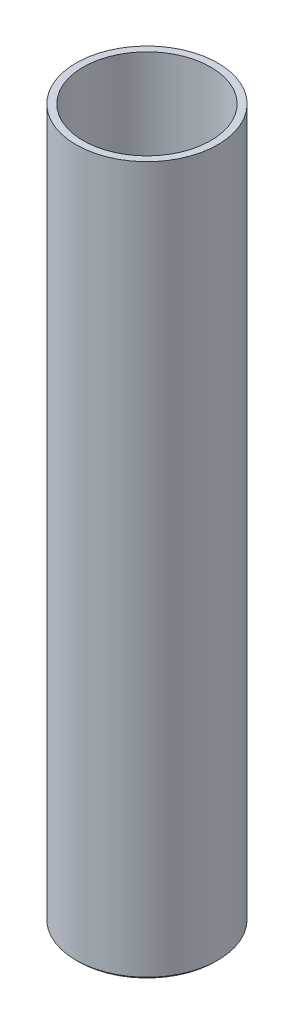
from build123d import *

# Parameters (mm, degrees)
SKETCH1_R           = 15
BOSS_EXTRUDE1_DEPTH = 150
SKETCH3_W           = 13.5
SKETCH3_H           = 147.5
SKETCH3_H_2         = 0.5
CHAMFER1_SIZE       = 0.5


with BuildPart() as part:
    # Sketch1 → Boss-Extrude1 (new body)
    with BuildSketch(Plane(origin=(0, 0, 0), x_dir=(1, 0, 0), z_dir=(0, 1, 0))):
        with Locations(Location((0, 0, 0), (0, 0, 270))):
            Circle(SKETCH1_R)
    extrude(amount=BOSS_EXTRUDE1_DEPTH)

    # Sketch3 → Cut-Revolve1 (revolve, cut)
    with BuildSketch(Plane.XY, mode=Mode.PRIVATE) as cut_revolve1_sk:
        with Locations((6.75, 76.25)):
            Rectangle(SKETCH3_W, SKETCH3_H)
        with Locations((6.75, 0.25)):
            Rectangle(SKETCH3_W, SKETCH3_H_2)
    revolve(cut_revolve1_sk.sketch.rotate(Axis((0, 0, 0), (0, 1, 0)), 90), axis=Axis((0, 0, 0), (0, 1, 0)), mode=Mode.SUBTRACT)

    # Chamfer1
    chamfer1_edges = [part.edges().sort_by_distance(p)[0] for p in [
        (0, 0, -15),
    ]]
    chamfer(chamfer1_edges, length=CHAMFER1_SIZE)


solid = part.part
